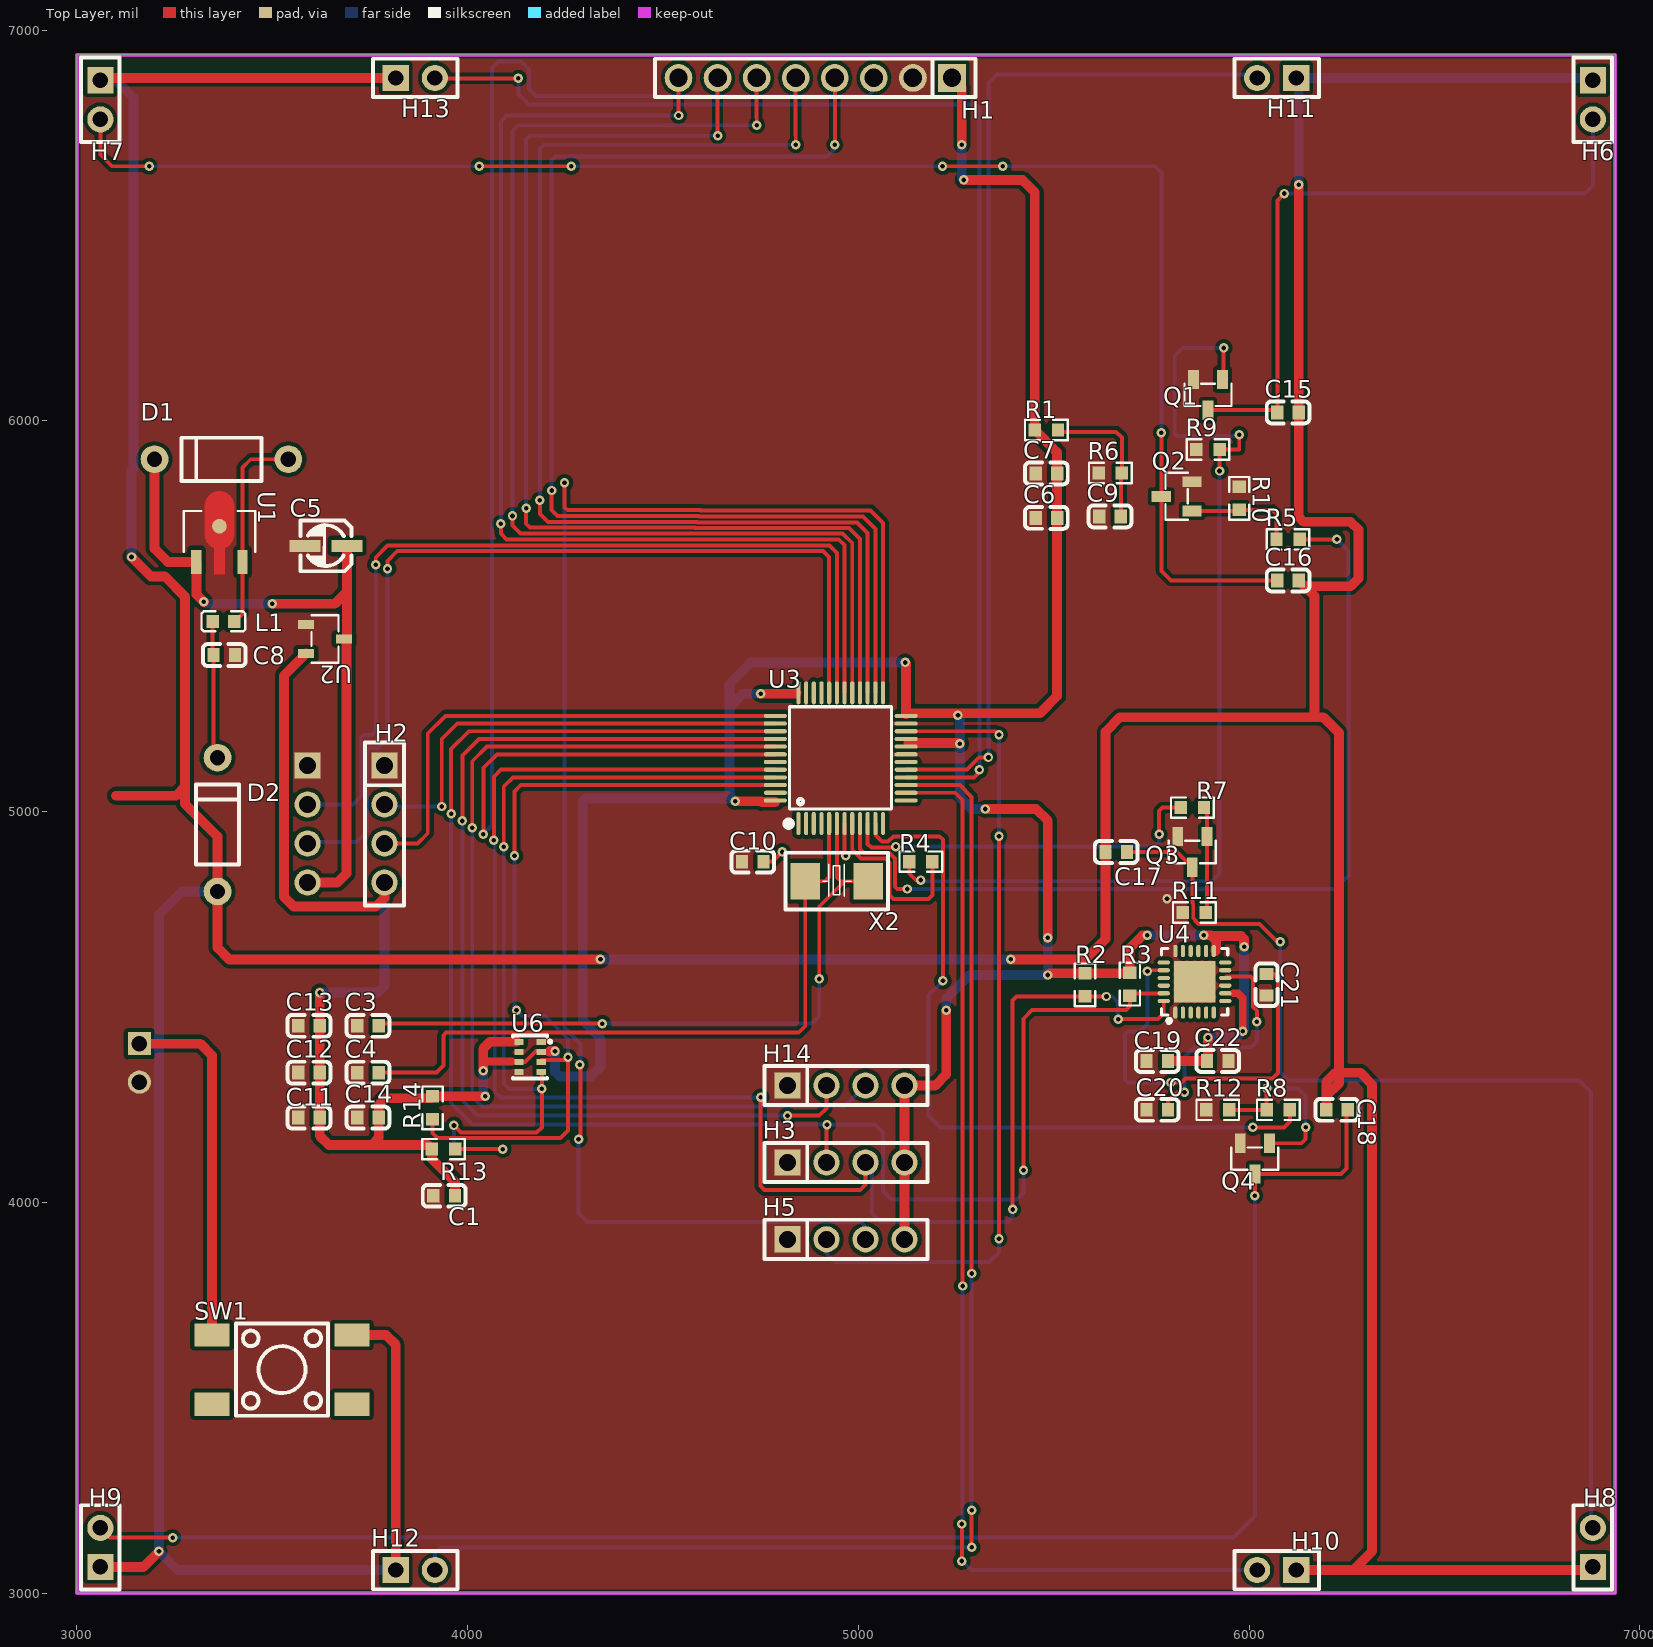
[diagram p0: Top Layer view]
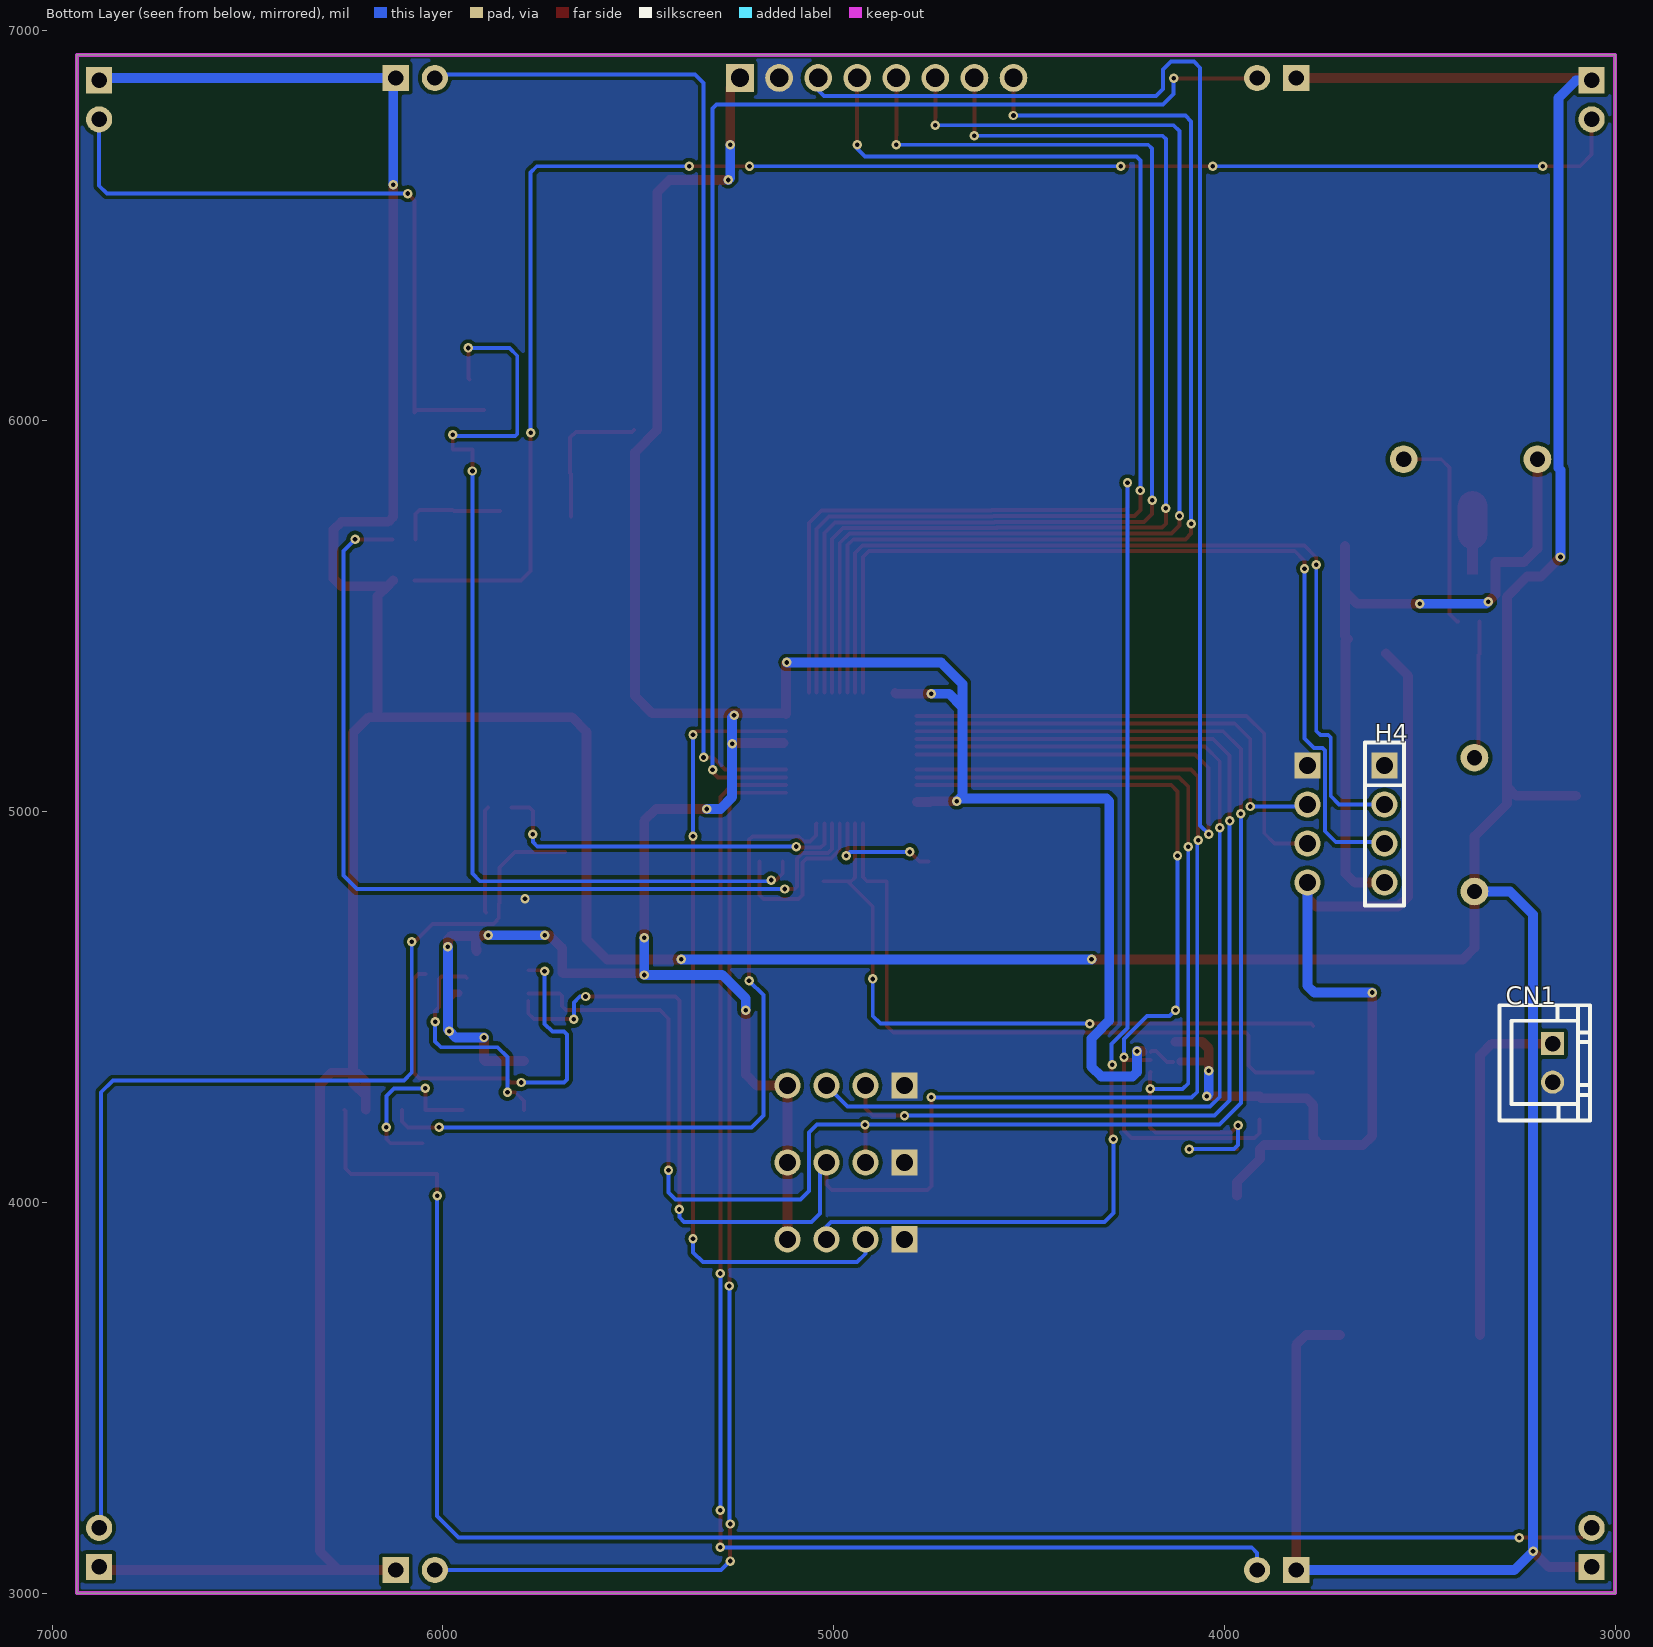
[diagram p1: Bottom Layer view, seen from below]
# Altium PCB MISC51791.pcbdoc
Units mil, origin at the board's own origin, x right, y up, seen from the top; angles counter-clockwise.
Board outline 3937.01 x 3937.01 mil, 2 copper layers (Top Layer, Bottom Layer), stack 62.206 mil thick; 64 components, 49 nets, 227 pads, 105 vias.

## Layer stack, top to bottom
Top Solder Mask Layer: solder mask 0.394, Dk 3.3
Top Layer: signal copper 1.379
Dielectric1: surface 59.449, FR4, Dk 4.5
Bottom Layer: signal copper 1.378
Bottom Solder Mask Layer: solder mask 0.394, Dk 3.3

## Board outline
3000,6937.01 3000,3000 6937.01,3000 6937.01,6937.01

## Design rules (kind name [scope] priority, off if disabled: settings)
BoardOutlineClearance copperThickness2oz_1 [All] p2 off: genericclearance=7.99 ignorepadtopadclearanceinfootprint=FALSE except(0: Arc-SplitContinuation Track-SplitContinuation SMDPad-SplitContinuation THPad-SplitContinuation Via-SplitContinuation Fill-SplitContinuation Region-SplitContinuation Poly-SplitContinuation Text-SplitContinuation Hole-SplitContinuation; 5.98: Arc-CutoutEdge SMDPad-CutoutEdge THPad-CutoutEdge Via-CutoutEdge Fill-CutoutEdge Region-CutoutEdge Text-CutoutEdge; 6.93: Hole-OutlineEdge Hole-CutoutEdge; 10: Poly-OutlineEdge Poly-CutoutEdge; 11.81: Arc-OutlineEdge Track-OutlineEdge SMDPad-OutlineEdge THPad-OutlineEdge Via-OutlineEdge Fill-OutlineEdge Region-OutlineEdge Text-OutlineEdge Track-CutoutEdge)
BoardOutlineClearance copperThickness1oz_1 [All] p4: genericclearance=4.02 ignorepadtopadclearanceinfootprint=FALSE except(0: Arc-SplitContinuation Track-SplitContinuation SMDPad-SplitContinuation THPad-SplitContinuation Via-SplitContinuation Fill-SplitContinuation Region-SplitContinuation Poly-SplitContinuation Text-SplitContinuation Hole-SplitContinuation; 6: SMDPad-CutoutEdge THPad-CutoutEdge Via-CutoutEdge Fill-CutoutEdge Region-CutoutEdge Text-CutoutEdge; 6.93: Hole-OutlineEdge Hole-CutoutEdge; 10: Poly-OutlineEdge Poly-CutoutEdge; 11.8: Arc-OutlineEdge Track-OutlineEdge SMDPad-OutlineEdge THPad-OutlineEdge Via-OutlineEdge Fill-OutlineEdge Region-OutlineEdge Text-OutlineEdge; 11.81: Arc-CutoutEdge Track-CutoutEdge)
Clearance copperThickness2oz [All] p1 off: gap=7.99 ignorepadtopadclearanceinfootprint=FALSE except(5.98: SMDPad-Track SMDPad-SMDPad THPad-Track SMDPad-THPad THPad-THPad Track-Via SMDPad-Via THPad-Via Via-Via Fill-Track Region-Track Fill-SMDPad Region-SMDPad Fill-THPad Region-THPad Fill-Via Region-Via Fill-Fill Fill-Region Region-Region Arc-Track Arc-SMDPad Arc-THPad Arc-Via Fill-Arc Region-Arc Arc-Arc Text-Track SMDPad-Text Text-THPad Text-Via Fill-Text Region-Text Arc-Text Text-Text; 6.93: Hole-Track Hole-SMDPad Hole-THPad Hole-Via Fill-Hole Region-Hole Hole-Arc Hole-Text; 10: Poly-Track Poly-SMDPad Poly-THPad Poly-Via Poly-Fill Poly-Region Poly-Poly Poly-Arc Poly-Text Poly-Hole)
Clearance copperThickness1oz [All] p3: gap=4.02 ignorepadtopadclearanceinfootprint=FALSE except(5.98: SMDPad-Track SMDPad-SMDPad THPad-Track SMDPad-THPad THPad-THPad Track-Via SMDPad-Via THPad-Via Via-Via Fill-Track Region-Track Fill-SMDPad Region-SMDPad Fill-THPad Region-THPad Fill-Via Region-Via Fill-Fill Fill-Region Region-Region; 6: Arc-Track Arc-SMDPad Arc-THPad Arc-Via Fill-Arc Region-Arc Arc-Arc Text-Track SMDPad-Text Text-THPad Text-Via Fill-Text Region-Text Arc-Text Text-Text; 6.93: Hole-Track Hole-SMDPad Hole-THPad Hole-Via Fill-Hole Region-Hole Hole-Arc Hole-Text; 10: Poly-Track Poly-SMDPad Poly-THPad Poly-Via Poly-Fill Poly-Region Poly-Poly Poly-Arc Poly-Text Poly-Hole)
DiffPairsRouting differentialPair [All] p1: maxlimit=6 minlimit=6 mostfreqgap=6 toplayer_minwidth=5 toplayer_prefwidth=10 toplayer_maxwidth=100 toplayer_mingap=6 toplayer_prefgap=6 toplayer_maxgap=6 bottomlayer_minwidth=5 bottomlayer_prefwidth=10 bottomlayer_maxwidth=100 bottomlayer_mingap=6 bottomlayer_prefgap=6 bottomlayer_maxgap=6 maxuncoupledlength=10
HoleToHoleClearance otherClearance [All] p1: gap=11.81 allowstackedmicrovias=TRUE
Length netLength [All] p1: minlimit=0 maxlimit=0
MatchedLengths netLengthTolerance [All] p1: tolerance=1000
PasteMaskExpansion pasteMaskExpansion [All] p1: expansion=0
PlaneConnect innerPlane [All] p1: planeconnectstyle=Relief reliefexpansion=20 reliefentries=4 reliefconductorwidth=10 reliefairgap=10
PolygonConnect "copperRegion_Top Layer" [(InNet('GND')) And OnLayer('Top Layer')] p1: connectstyle=Direct reliefconductorwidth=10 reliefentries=4 polygonreliefangle="90 Angle" airgapwidth=10 via.connectstyle=Relief via.reliefconductorwidth=10 via.reliefentries=4 via.polygonreliefangle="90 Angle" via.airgapwidth=10
PolygonConnect "copperRegion_Bottom Layer" [(InNet('GND')) And OnLayer('Bottom Layer')] p2: connectstyle=Direct reliefconductorwidth=10 reliefentries=4 polygonreliefangle="90 Angle" airgapwidth=10 via.connectstyle=Relief via.reliefconductorwidth=10 via.reliefentries=4 via.polygonreliefangle="90 Angle" via.airgapwidth=10
PolygonConnect copperRegion [(InNet('GND'))] p3: connectstyle=Direct reliefconductorwidth=10 reliefentries=4 polygonreliefangle="90 Angle" airgapwidth=10 via.connectstyle=Relief via.reliefconductorwidth=10 via.reliefentries=4 via.polygonreliefangle="90 Angle" via.airgapwidth=10
RoutingVias viaSize [All] p1: holewidth=12.01 width=24.02 viastyle="Through Hole" minholewidth=11.81 minwidth=19.68 maxholewidth=248.03 maxwidth=393.7
SolderMaskExpansion solderMaskExpansion [IsVia] p1: expansion=-1000 istentingtop=TRUE
SolderMaskExpansion solderMaskExpansion [All] p2: expansion=2 istentingtop=FALSE
Width copperThickness2oz_2 [All] p1 off: maxlimit=100 minlimit=8 preferedwidth=10
Width copperThickness1oz_2 [All] p2: maxlimit=100 minlimit=5 preferedwidth=10

## Components (designator, comment, footprint, x,y, rotation, side; value= is the part's Value field where it differs from the comment)
C1 "100nF" C0603 3940,4017.01 r0 top
C3 "20pF" C0603 3745,4452.01 r0 top
C4 "20pF" C0603 3745,4332.01 r0 top
C5 "0.1uF" C_Ele_SMD_3x5.4mm 3637.34,5680.81 r0 top
C6 "0.1uF" C0603 5481.33,5752.01 r0 top
C7 "0.1uF" C0603 5481.33,5865.81 r0 top
C8 "0.1uF" C0603 3377.29,5400.81 r180 top
C9 "22pF" C0603 5644.34,5755.81 r0 top
C10 "0.1uF" C0603 4730,4872.01 r0 top
C11 "0.1uF" C0603 3593.97,4217.01 r0 top
C12 "0.1uF" C0603 3593.97,4332.15 r0 top
C13 "0.1uF" C0603 3593.97,4452.01 r0 top
C14 "0.1uF" C0603 3745,4217.01 r0 top
C15 "0.1uF" C0603 6100,6022.01 r0 top
C16 "0.1uF" C0603 6100,5592.01 r0 top
C17 "0.1uF" C0603 5660,4897.01 r180 top
C18 "0.1uF" C0603 6225,4237.01 r180 top
C19 "10nF" C0603 5765.21,4361.95 r0 top
C20 "0.1uF" C0603 5765,4237.01 r0 top
C21 "2.2nF" C0603 6045,4557.01 r270 top
C22 "0.1uF" C0603 5920,4362.01 r0 top
CN1 "HX-XH2.54-2PZZ" CONN-TH_2P-P2.50_HX-2.54MM-2P-ZZ-MS 3160,4357.01 r270 bottom
D1 "" DO_1N4007 3370,5902.01 r0 top
D2 "" DO_1N4007 3360,4967.01 r270 top
H1 "" HDR-TH_8P-P2.54-V-F-1 4889.76,6877.95 r180 top
H2 "" HDR-TH_4P-P2.54-V-F 3787.4,4968.5 r270 top
H3 "" HDR-TH_4P-P2.54-V-F 4968.5,4102.38 r0 top
H4 "" HDR-TH_4P-P2.54-V-F 3590.55,4968.5 r270 bottom
H5 "" HDR-TH_4P-P2.54-V-F 4968.5,3905.53 r0 top
H6 "" HDR-TH_2P-P2.54-V-F 6880,6822.01 r270 top
H7 "" HDR-TH_2P-P2.54-V-F 3060,6822.01 r270 top
H8 "" HDR-TH_2P-P2.54-V-F 6880,3117.01 r90 top
H9 "" HDR-TH_2P-P2.54-V-F 3060,3117.01 r90 top
H10 "" HDR-TH_2P-P2.54-V-F 6070.86,3059.07 r180 top
H11 "" HDR-TH_2P-P2.54-V-F 6070.87,6877.95 r180 top
H12 "" HDR-TH_2P-P2.54-V-F 3866.14,3059.06 r0 top
H13 "" HDR-TH_2P-P2.54-V-F 3866.14,6877.95 r0 top
H14 "" HDR-TH_4P-P2.54-V-F 4968.5,4299.21 r0 top
L1 "47uH" L0603 3375,5487.01 r0 top
Q1 "" SOT-23-3_L2.9-W1.3-P1.90-LS2.4-BR 5895,6067.01 r90 top
Q2 "" SOT-23-3_L2.9-W1.3-P1.90-LS2.4-BR 5815,5807.01 r0 top
Q3 "" SOT-23-3_L2.9-W1.3-P1.90-LS2.4-BR 5855,4897.01 r90 top
Q4 "" SOT-23-3_L2.9-W1.3-P1.90-LS2.4-BR 6015,4112.01 r90 top
R1 "100R" R0603 5481.33,5977.01 r180 top
R2 "4.7K" R0603 5580,4557.01 r90 top
R3 "4.7K" R0603 5694.92,4558.62 r90 top
R4 "100R" R0603 5160,4872.01 r0 top locked
R5 "100R" R0603 6100,5697.01 r0 top
R6 "100R" R0603 5645,5867.01 r0 top
R7 "100R" R0603 5855.02,5010.49 r180 top
R8 "100R" R0603 6075,4237.01 r0 top
R9 "10K" R0603 5895,5927.01 r0 top
R10 "10K" R0603 5975,5802.01 r270 top
R11 "10K" R0603 5860,4742.01 r0 top
R12 "10K" R0603 5920,4237.01 r0 top
R13 "4.7K" R0603 3938.37,4136.44 r180 top
R14 "4.7K" R0603 3910,4242.01 r90 top
SW1 "KH-6X6X5H-STM" SW-SMD_4P-L6.0-W6.0-P4.50-LS9.0_H5.0 3525,3572.01 r0 top
U1 "78L05" SOT-89-3_L4.5-W2.5-P1.50-LS4.2-BR 3364.91,5692.7 r270 top
U2 "XC6206P332MR-G" SOT-23-3_L2.9-W1.6-P1.90-LS2.8-BR 3635,5442.01 r180 top
U3 "STM32G474CBT6" LQFP-48_L7.0-W7.0-P0.50-LS9.0-BL 4955,5137.01 r0 top locked
U4 "MPU-6050" QFN-24_L4.0-W4.0-P0.50-BL-EP2.7 5860.53,4564.7 r0 top
U6 "BMP280" LGA-8_L2.5-W2.0-P0.65_AMP6127 4160,4372.01 r0 top
X2 "8MHz" CRYSTAL-SMD_L5.0-W3.2 4945,4822.01 r180 top

## Footprints (in the part's own frame and the unit in brackets; to place one, negate y for a bottom-side part, rotate by r counter-clockwise, add the part's x,y. Pads: shape width x height; smd on the part's side, far side on the other; paste and mask are expansions set on the pad)
C0603 [mm]
  rect 0.8x0.9 smd: 1(-0.7,0) 2(0.7,0)
  silkscreen extent -1.39,-0.71 1.39,0.71
C_Ele_SMD_3x5.4mm [mil]
  rect 78.7x31.5 smd paste+0 mask+2: 1(54.1,-0.55) 2(-53.7,-0.55)
  silkscreen extent -65,-65 65,65
CONN-TH_2P-P2.50_HX-2.54MM-2P-ZZ-MS [mm]
  rect 1.5x1.5 hole 1: 1(-1.25,0)
  round 1.5 hole 1: 2(1.25,0)
  silkscreen extent -3.75,-3.46 3.75,2.44
CRYSTAL-SMD_L5.0-W3.2 [mm]
  rect 1.9x2.4 smd: 1(-2.05,0) 2(2.05,0)
  silkscreen extent -3.32,-1.85 3.33,1.85
DO_1N4007 [mm]
  round 1.8 hole 1 paste+0 mask+0.051: 1(-4.35,0) 2(4.35,0)
  silkscreen extent -2.6,-1.4 2.6,1.4
HDR-TH_2P-P2.54-V-F [mm]
  rect 1.7x1.7 hole 1: 1(-1.27,0)
  round 1.7 hole 1: 2(1.27,0)
  silkscreen extent -2.74,-1.25 2.74,1.25
HDR-TH_4P-P2.54-V-F [mm]
  rect 1.7x1.7 hole 1.1: 1(-3.81,0)
  round 1.7 hole 1.1: 2(-1.27,0) 3(1.27,0) 4(3.81,0)
  silkscreen extent -5.29,-1.27 5.29,1.27
HDR-TH_8P-P2.54-V-F-1 [mm]
  rect 1.8x1.8 hole 1.2: 1(-8.89,0)
  round 1.8 hole 1.2: 2(-6.35,0) 3(-3.81,0) 4(-1.27,0) 5(1.27,0) 6(3.81,0) 7(6.35,0) 8(8.89,0)
  silkscreen extent -10.41,-1.25 10.41,1.25
L0603 [mm]
  rect 0.8x0.864 smd paste-100 mask+0.051: 1(-0.7,0) 2(0.7,0)
  silkscreen extent -1.42,-0.65 1.42,0.65
LGA-8_L2.5-W2.0-P0.65_AMP6127 [mm]
  rect 0.6x0.4 smd: 1(0.725,0.975) 2(0.725,0.325) 3(0.725,-0.325) 4(0.725,-0.975) 5(-0.725,-0.975) 6(-0.725,-0.325) 7(-0.725,0.325) 8(-0.725,0.975)
  silkscreen extent -1.1,-1.4 1.4,1.4
LQFP-48_L7.0-W7.0-P0.50-LS9.0-BL [mm]
  oval 0.27x1.5 smd paste+0 mask+0.05: 1(-2.75,-4.25) 2(-2.25,-4.25) 3(-1.75,-4.25) 4(-1.25,-4.25) 5(-0.75,-4.25) 6(-0.25,-4.25) 7(0.25,-4.25) 8(0.75,-4.25) 9(1.25,-4.25) 10(1.75,-4.25) 11(2.25,-4.25) 12(2.75,-4.25) 25(2.75,4.25) 26(2.25,4.25) 27(1.75,4.25) 28(1.25,4.25) 29(0.75,4.25) 30(0.25,4.25) 31(-0.25,4.25) 32(-0.75,4.25) 33(-1.25,4.25) 34(-1.75,4.25) 35(-2.25,4.25) 36(-2.75,4.25)
  oval 1.5x0.27 smd paste+0 mask+0.05: 13(4.25,-2.75) 14(4.25,-2.25) 15(4.25,-1.75) 16(4.25,-1.25) 17(4.25,-0.75) 18(4.25,-0.25) 19(4.25,0.25) 20(4.25,0.75) 21(4.25,1.25) 22(4.25,1.75) 23(4.25,2.25) 24(4.25,2.75) 37(-4.25,2.75) 38(-4.25,2.25) 39(-4.25,1.75) 40(-4.25,1.25) 41(-4.25,0.75) 42(-4.25,0.25) 43(-4.25,-0.25) 44(-4.25,-0.75) 45(-4.25,-1.25) 46(-4.25,-1.75) 47(-4.25,-2.25) 48(-4.25,-2.75)
  silkscreen extent -3.59,-4.46 3.3,3.34
QFN-24_L4.0-W4.0-P0.50-BL-EP2.7 [mm]
  oval 0.28x0.8 smd paste-100 mask+0.05: 1(-1.25,-2) 2(-0.75,-2) 3(-0.25,-2) 4(0.25,-2) 5(0.75,-2) 6(1.25,-2) 13(1.25,2) 14(0.75,2) 15(0.25,2) 16(-0.25,2) 17(-0.75,2) 18(-1.242,2)
  oval 0.8x0.28 smd paste-100 mask+0.05: 7(2,-1.25) 8(2,-0.75) 9(2,-0.25) 10(2,0.25) 11(2,0.75) 12(2,1.25) 19(-2,1.25) 20(-2,0.75) 21(-2,0.25) 22(-2,-0.25) 23(-2,-0.75) 24(-2,-1.25)
  rect 2.7x2.7 smd paste-100 mask+0.05: 25(0.012,0)
  silkscreen extent -2.14,-2.79 2.16,2.15
R0603 [mil]
  rect 31.75x34.02 smd paste-3937.01 mask+2: 1(-29.66,0) 2(29.66,0)
  silkscreen extent -55,-26 55,26
SOT-23-3_L2.9-W1.3-P1.90-LS2.4-BR [mm]
  rect 1.25x0.7 smd: 1(1,-0.95) 2(1,0.95) 3(-1,0)
  silkscreen extent -0.73,-1.53 0.73,1.53
SOT-23-3_L2.9-W1.6-P1.90-LS2.8-BR [mm]
  rect 1.07x0.6 smd: 1(1.235,-0.95) 2(1.235,0.95) 3(-1.235,0)
  silkscreen extent -0.88,-1.54 0.88,1.54
SOT-89-3_L4.5-W2.5-P1.50-LS4.2-BR [mm]
  rect 1.575x0.672 smd: 1(1.356,-1.5) 3(1.356,1.5)
  round 0.95 smd: 2(-0.966,0)
  Top Layer region: -2.283,0.95 -0.429,0.95 -0.384,0.949 -0.34,0.946 -0.296,0.94 -0.252,0.933 -0.208,0.924 -0.165,0.912 -0.123,0.899 -0.081,0.884 -0.04,0.866 0,0.847 0.04,0.826 0.078,0.803 0.115,0.779 0.151,0.752 0.185,0.724 0.219,0.695 0.251,0.664 0.281,0.631 0.31,0.597 0.337,0.562 0.362,0.525 0.386,0.488 0.408,0.449 0.428,0.409 0.447,0.33 2.144,0.33 2.144,-0.33 0.447,-0.33 0.428,-0.409 0.408,-0.449 0.386,-0.488 0.362,-0.526 0.337,-0.562 0.31,-0.597 0.281,-0.631 0.251,-0.664 0.219,-0.695 0.185,-0.725 0.151,-0.753 0.115,-0.779 0.078,-0.804 0.04,-0.827 0,-0.848 -0.04,-0.867 -0.081,-0.884 -0.123,-0.899 -0.165,-0.913 -0.208,-0.924 -0.252,-0.934 -0.296,-0.941 -0.34,-0.946 -0.384,-0.949 -0.429,-0.95 -2.283,-0.95 -2.328,-0.949 -2.372,-0.946 -2.416,-0.941 -2.46,-0.934 -2.504,-0.924 -2.547,-0.913 -2.589,-0.899 -2.631,-0.884 -2.672,-0.867 -2.713,-0.848 -2.752,-0.827 -2.79,-0.804 -2.827,-0.779 -2.863,-0.753 -2.898,-0.725 -2.931,-0.695 -2.963,-0.664 -2.993,-0.631 -3.022,-0.597 -3.049,-0.562 -3.075,-0.526 -3.098,-0.488 -3.12,-0.449 -3.141,-0.409 -3.159,-0.369 -3.175,-0.327 -3.189,-0.285 -3.202,-0.242 -3.212,-0.199 -3.22,-0.155 -3.227,-0.111 -3.231,-0.067 -3.233,-0.022 -3.233,0.022 -3.231,0.067 -3.227,0.111 -3.22,0.155 -3.212,0.199 -3.202,0.242 -3.189,0.285 -3.175,0.327 -3.159,0.369 -3.141,0.409 -3.12,0.449 -3.098,0.488 -3.075,0.525 -3.049,0.562 -3.022,0.597 -2.993,0.631 -2.963,0.664 -2.931,0.695 -2.898,0.724 -2.863,0.752 -2.827,0.779 -2.79,0.803 -2.752,0.826 -2.713,0.847 -2.672,0.866 -2.631,0.884 -2.589,0.899 -2.547,0.912 -2.504,0.924 -2.46,0.933 -2.416,0.94 -2.372,0.946 -2.328,0.949
  silkscreen extent -1.95,-2.33 0.7,2.33
SW-SMD_4P-L6.0-W6.0-P4.50-LS9.0_H5.0 [mm]
  rect 2.3x1.5 smd: 1(-4.55,2.25) 2(4.55,2.25) 3(-4.55,-2.25) 4(4.55,-2.25)
  silkscreen extent -3,-3 3,3

## Via types
v1: diameter 24.02, hole 12, Top Layer to Bottom Layer, 105 vias

## Nets (pads, with @x,y where several pads share a name; then routed paths per layer and width w, separated by ;. In a path a pad name is that pad's centre, name@x,y a point inside that pad or via, vN(x,y) a via of type N, cw(c..) or ccw(c..) an arc to the next point about the centre after c; other vN are vias at no path point)
3.3V: C1.2 C6.2 C7.2 C11.2 C12.2 C13.2 C14.2 C19.2 C22.1 H1.1 H2.4 H3.4 H5.4 H14.4 R1.2 R2.2 R3.2 R13.2 R14.2 U2.2 U3.20 U3.21 U3.24 U3.36 U3.48 U4.8 U4.13 U6.2 U6.6 U6.8 | length 10851.4
  Top Layer w10: U6.6 4147.21,4359.22 4175,4387.01 4186.33,4387.01 U6.2 ; C22.1 C22.1@5895,4364.57
  Top Layer w20: 4040,4358.91 4042.03,4360.94 4112.96,4360.94 ; 5960.22,4535.17 5971.83,4535.17 5983.79,4523.22 v1(5983.79,4438.22)
  Top Layer w25: U2.2 3530,5348.23 3530,4782.01 3555,4757.01 3765,4757.01 3787.4,4779.41 H2.4 ; v1(3621.53,4537.01) C13.2 C12.2 C11.2 3621.53,4170.47 3645,4147.01 3755,4147.01 ; C1.2 3967.56,4052.36 3908.71,4111.21 R13.2 3898.14,4147.01 3755,4147.01 ; v1@4040,4271.67 R14.2 3905,4266.67 3789.66,4266.67 3772.56,4249.57 C14.2 3772.56,4164.57 3755,4147.01 ; v1(4040,4337.01) 4040,4358.91 4040,4393.48 4057.68,4411.16 U6.8@4125.18,4411.16 ; 4209.65,4385.68 4211.18,4387.21 v1(4223.8,4387.21) ; v1(4685,5027.01) 4751.23,5027.01 4753.61,5024.63 U3.48@4787.68,5024.63 ; v1(4750,5302.01) 4840.3,5302.01 U3.36@4842.62,5304.33 ; H5.4 H3.4 H14.4 5197.2,4299.21 5225,4327.01 v1(5225,4492.01) ; v1(5120,5382.01) 5122.32,5379.69 U3.24@5122.32,5250.28 ; U3.24@5122.32,5249.39 U3.24@5122.32,5250.28 ; 5128.44,5175.99 5257.62,5175.99 v1(5260,5173.61) ; H1.1 5265,6852.72 v1(5265,6707.01) ; v1(5270,6617.01) 5420,6617.01 5451.67,6585.34 R1.2 5508.89,5919.79 C7.2 C6.2 5508.89,5295.9 5465,5252.01 5260,5252.01 v1(5255,5247.01) 5250,5252.01 5124.05,5252.01 U3.24@5122.32,5250.28 ; v1(5325,5007.01) 5455,5007.01 5485,4977.01 v1(5485,4677.01) ; v1(5485,4582.01) 5489.66,4586.67 R2.2 5693.31,4586.67 R3.2 5694.92,4651.58 5726.82,4683.48 v1(5739.61,4683.48) ; C19.2 C22.1 ; v1(5884.09,4683.48) 5903.52,4683.48 5909.74,4677.27 ; C22.1@5895,4364.57 v1(5895,4422.01) ; U4.13@5914.06,4643.44 5914.06,4647.76 5915.97,4649.67 5915.97,4671.03 5909.74,4677.27 ; v1(5987.5,4654.51) 5987.5,4674.51 5980,4682.01 5914.48,4682.01 5909.74,4677.27
  Bottom Layer w25: v1(3621.53,4537.01) 3770,4537.01 3787.4,4554.41 H2.4 ; v1(4040,4337.01) 4040,4276.67 v1(4045,4271.67) ; v1(4223.8,4387.21) 4223.8,4333.21 4235,4322.01 4315,4322.01 4340,4347.01 4340,4419.37 4314.51,4444.86 4314.51,4446.27 4295,4465.78 4295,5027.01 4302.07,5034.08 v1@4677.93,5034.08 ; v1(4685,5027.01) v1@4677.93,5034.08 ; v1(4750,5302.01) 4705,5302.01 4671.08,5268.09 4670,5268.09 ; v1(5120,5382.01) 4725,5382.01 4670,5327.01 4670,5268.09 ; v1(5225,4492.01) 5225,4522.01 5285,4582.01 v1(5485,4582.01) v1(5485,4677.01) ; v1(5255,5247.01) 5260,5242.01 v1(5260,5173.61) 5260,5037.01 5290,5007.01 v1(5325,5007.01) ; v1(5265,6707.01) 5265,6622.01 v1(5270,6617.01) ; v1(5739.61,4683.48) v1(5884.09,4683.48) ; v1(5895,4422.01) 5967.57,4422.01 v1(5983.79,4438.22) 5987.5,4441.93 v1(5987.5,4654.51) ; 4670,5268.09 4670,5042.01 v1@4677.93,5034.08
$1N3: C8.2 D2.1 L1.1 | length 353.9
  Top Layer w10: L1.1 3347.45,5403.1 C8.2 3349.73,5148.53 D2.1
$1N6: D1.2 L1.2 U1.3 | length 530.3
  Top Layer w10: L1.2 3405,5487.01 3423.96,5505.97 U1.3 3423.96,5880.97 3445,5902.01 D1.2
$1N10: C9.2 R1.1 R6.2 | length 374.5
  Top Layer w10: R1.1 5515.99,5972.01 5660,5972.01 5674.66,5957.35 R6.2 5671.9,5864.25 C9.2
$1N18: C10.2 U3.7 | length 309.3
  Top Layer w10: C10.2 4780,4872.01 v1(4805,4897.01) ; U3.7 4964.84,4890.21 v1(4968.15,4886.9)
  Bottom Layer w10: v1(4805,4897.01) 4958.04,4897.01 v1(4968.15,4886.9)
$1N84: C15.1 H6.2 Q1.3 | length 1715.3
  Top Layer w10: Q1.3 6066.81,6027.64 C15.1 6072.44,6564.45 v1(6090,6582.01)
  Bottom Layer w10: v1(6090,6582.01) 6860,6582.01 6880,6602.01 H6.2
$1N86: Q1.1 R4.1 R9.2 | length 2597.8
  Top Layer w10: R4.1 5130.34,4841.67 5147.01,4825 v1(5160,4825) ; v1(5924.66,5872.01) R9.2 5975,5927.01 v1(5975,5964.94) ; Q1.1 5935,6108.98 v1(5935,6187.01)
  Bottom Layer w10: v1(5160,4825) 5162.99,4822.01 5905,4822.01 5924.66,4841.67 v1(5924.66,5872.01) ; v1(5935,6187.01) 5830,6187.01 5810,6167.01 5810,5967.01 5815,5962.01 5972.07,5962.01 v1(5975,5964.94)
$1N89: Q2.1 R5.1 R10.2 | length 286.2
  Top Layer w10: Q2.1 5972.26,5769.61 R10.2 6059.66,5772.35 6070.34,5761.67 R5.1
$1N91: C16.1 H7.2 Q2.3 | length 4151.4
  Top Layer w10: H7.2 3060,6682.01 3090,6652.01 v1(3185,6652.01) ; v1(4030,6652.01) v1(4265,6652.01) ; v1(5215.44,6652.01) v1(5370,6652.01) ; v1(5775.63,5970.18) Q2.3 5775.63,5616.38 5800,5592.01 C16.1
  Bottom Layer w10: v1(3185,6652.01) v1(4030,6652.01) ; v1(4265,6652.01) v1(5215.44,6652.01) ; v1(5370,6652.01) 5760,6652.01 5775.63,6636.38 v1(5775.63,5970.18)
$1N94: Q3.1 R7.1 R11.2 | length 272.8
  Top Layer w10: R7.1 5892.4,5002.77 Q3.1 5892.4,4744.75 R11.2
$1N96: C17.1 H8.2 Q3.3 | length 2831.3
  Top Layer w10: C17.1 5815.63,4897.01 Q3.3 5855,4765.77 5857.2,4763.57 5857.2,4727.83 5862.8,4722.23 5862.8,4720.45 5871.02,4712.23 6027.29,4712.23 6072.52,4667.01 v1(6080,4667.01)
  Bottom Layer w10: v1(6080,4667.01) 6080,4332.01 6100,4312.01 6845,4312.01 6875,4282.01 6875,3172.01 H8.2
$1N99: Q4.1 R8.1 R12.2 | length 466.1
  Top Layer w10: R12.2 R8.1 6045,4237.35 v1(6045,4292.01) ; Q4.1 6134.37,4151.38 6145,4162.01 v1(6145,4192.01)
  Bottom Layer w10: v1(6045,4292.01) 6125,4292.01 6145,4272.01 v1(6145,4192.01)
$1N101: C18.1 H9.2 Q4.3 | length 4255.8
  Top Layer w10: H9.2 3085,3142.01 v1(3245,3142.01) ; v1(6015,4017.01) Q4.3 6235.63,4072.64 6250,4087.01 6250,4234.45 C18.1
  Bottom Layer w10: v1(3245,3142.01) 5960,3142.01 6015,3197.01 v1(6015,4017.01)
$1N107: C20.2 U4.10 | length 604.4
  Top Layer w10: C20.2 5792.56,4259.57 5815,4282.01 v1(5835,4282.01) ; U4.10 5942.46,4577.73 6004.28,4577.73 6010,4572.01 6010,4500.45 6020,4490.45 v1(6020,4462.01)
  Bottom Layer w10: v1(5835,4282.01) 5835,4372.01 5860,4397.01 6005,4397.01 6020,4412.01 v1(6020,4462.01)
$1N110: C21.1 U4.20 | length 1041.3
  Top Layer w10: v1(5740,4592.01) 5744.85,4592.01 5747.07,4594.23 U4.20 ; v1(5800,4307.01) 5827.48,4307.01 5837.48,4317.01 6060,4317.01 6073.7,4330.71 6073.7,4573.31 6062.44,4584.57 C21.1
  Bottom Layer w10: v1(5740,4592.01) 5740,4457.01 5720,4437.01 5690,4437.01 5682.93,4429.94 5682.93,4314.08 5690,4307.01 v1(5800,4307.01)
$1N126: C4.2 U3.5 X2.2 | length 1759.8
  Top Layer w10: C4.2 3920,4332.01 3937.93,4349.94 3937.93,4427.19 3945.24,4434.5 4847.49,4434.5 4864.29,4451.3 X2.2 4915,4822 4925.47,4832.48 U3.5
$1N129: C3.2 U3.6 X2.1 | length 1793.2
  Top Layer w10: C3.2 3778.04,4457.49 v1(4345,4457.49) ; v1(4900,4572.01) 4900,4757.54 4964.47,4822 X2.1 4955,4822.01 4945.16,4831.85 U3.6
  Bottom Layer w10: v1(4345,4457.49) 4880.48,4457.49 4900,4477.01 v1(4900,4572.01)
+5V: C5.1 D1.1 H4.4 U1.1 U2.3 | length 1794.4
  Top Layer w25: D1.1 3198.74,5673.27 3232.7,5639.31 U1.1 3305.85,5556.16 v1(3325,5537.01) ; v1(3500,5532.01) 3660,5532.01 3683.62,5555.63 ; H4.4 3666.5,4818.5 3690,4842.01 3690,5435.63 U2.3 3691.05,5449.43 3691.05,5555.63 3683.62,5555.63 ; C5.1 3691.44,5563.45 3683.62,5555.63
  Bottom Layer w25: v1(3325,5537.01) 3330,5532.01 v1(3500,5532.01)
CE: H1.3 U3.42 | length 3990.3
  Top Layer w10: v1(4040.1,4942.4) 4040.49,4942.79 4040.49,5112.5 4074.84,5146.85 U3.42
  Bottom Layer w10: v1(4040.1,4942.4) 4062.01,4964.31 4062.01,6904.02 4078.2,6920.21 4136.8,6920.21 4157.56,6899.45 4157.56,6849.45 4175.47,6831.54 5024.53,6831.54 5039.76,6846.77 H1.3
CSN: H1.4 U3.26 | length 3081.3
  Top Layer w10: v1(4215,5822.01) 4215,5772.01 4230,5757.01 4590.9,5757.01 4592.87,5755.04 5011.97,5755.04 5043.58,5723.43 U3.26 ; H1.4 4940,6877.72 v1(4940,6707.01)
  Bottom Layer w10: v1(4215,5822.01) 4215,6667.01 4225,6677.01 4920,6677.01 4940,6697.01 v1(4940,6707.01)
GND: C1.1 C3.1 C4.1 C5.2 C6.1 C7.1 C8.1 C9.1 C10.1 C11.1 C12.1 C13.1 C14.1 C19.1 C20.1 C21.2 C22.2 CN1.2 H1.2 H2.1 H3.1 H4.1 H5.1 H14.1 Q1.2 Q2.2 Q3.2 Q4.2 R6.1 R9.1 R10.1 R11.1 R12.1 U1.2 U2.1 U3.19 U3.23 U3.35 U3.47 U4.1 U4.9 U4.11 U4.18 U4.25 U6.1 U6.5 U6.7
  other v1: 5790,4777.01
IRQ: H1.8 U3.30 | length 2882.3
  Top Layer w10: v1(4085,5737.01) 4085,5712.01 4100,5697.01 4950,5697.01 4964.84,5682.17 U3.30 ; H1.8 4539.76,6806.77 4540,6806.54 v1(4540,6782.01)
  Bottom Layer w10: v1(4085,5737.01) 4085,6767.01 4100,6782.01 v1(4540,6782.01)
LED_PWM1: H10.2 U3.14 | length 2866.5
  Top Layer w10: U3.14 5248.58,5048.43 5267.01,5030 v1(5267.01,3786.07) ; v1(5265,3082.01) v1(5265,3177.01)
  Bottom Layer w10: v1(5265,3082.01) 5287.94,3059.07 H10.2 ; v1(5265,3177.01) 5267.01,3179.02 v1(5267.01,3786.07)
LED_PWM2: H11.2 U3.17 | length 2650.5
  Top Layer w10: U3.17 5277.95,5107.48 5309.34,5138.87 v1(5332.99,5138.87)
  Bottom Layer w10: v1(5332.99,5138.87) 5332.99,6865 5355,6887.01 6011.81,6887.01 H11.2
LED_PWM3: H12.2 U3.15 | length 3524.9
  Top Layer w10: U3.15 5260,5068.11 5290,5038.11 v1(5290,3817.89) ; v1(5290,3117.01) v1(5290,3212.01)
  Bottom Layer w10: H12.2 3916.14,3103.15 3930,3117.01 v1(5290,3117.01) ; v1(5290,3212.01) v1(5290,3817.89)
LED_PWM4: H13.2 U3.16 | length 3341.1
  Top Layer w10: H13.2 3917.09,6877.01 v1(4130,6877.01) ; U3.16 5295.79,5087.8 5310,5102.01 v1(5310,5107.01)
  Bottom Layer w10: v1(4130,6877.01) 4130,6837.01 4157.01,6810 5300,6810 5310,6800 v1(5310,5107.01)
MISO: H1.7 U3.28 | length 2890.3
  Top Layer w10: v1(4150,5777.01) 4150,5737.01 4160,5727.01 4581.53,5727.01 4582.51,5726.02 4975.98,5726.02 5004.21,5697.8 U3.28 ; H1.7 4639.76,6746.77 4640,6746.54 v1(4640,6730)
  Bottom Layer w10: v1(4150,5777.01) 4150,6722.01 4157.99,6730 v1(4640,6730)
MOSI: H1.6 U3.29 | length 3033.4
  Top Layer w10: v1(4115,5757.01) 4115,5732.01 4135,5712.01 4960,5712.01 4984.53,5687.48 U3.29 ; H1.6 4739.76,6776.77 4740,6776.54 v1(4740,6757.01)
  Bottom Layer w10: v1(4115,5757.01) 4115,6742.01 4130,6757.01 v1(4740,6757.01)
PWM1: R4.2 U3.8 | length 462.1
  Top Layer w10: U3.8 4984.53,4903.04 5007.33,4880.23 5070,4880.23 5080,4870.23 5080,4787.01 5090,4777.01 5180,4777.01 5189.66,4786.67 R4.2
PWM2: R5.2 U3.9 | length 2383
  Top Layer w10: U3.9 5004.21,4904.25 5014.21,4894.25 5079.79,4894.25 5094.02,4880.02 5094.02,4807.99 5100,4802.01 v1(5125,4802.01) ; R5.2 v1(6225,5697.01)
  Bottom Layer w10: v1(5125,4802.01) 6220,4802.01 6255,4837.01 6255,5667.01 v1(6225,5697.01)
PWM3: R7.2 U3.10 | length 946.5
  Top Layer w10: U3.10 5023.9,4917.76 5033.39,4908.26 5093.33,4908.26 v1(5095.81,4910.75) ; v1(5770,4942.01) 5770,5002.01 5778.48,5010.49 R7.2
  Bottom Layer w10: v1(5095.81,4910.75) 5758.74,4910.75 5770,4922.01 v1(5770,4942.01)
PWM4: R8.2 U3.11 | length 1913.1
  Top Layer w10: U3.11 5045,4968.27 5045,4939.56 5060.82,4923.74 5076.29,4923.74 5089.56,4937.01 5208.16,4937.01 5216.58,4928.59 v1(5216.58,4567.01) ; v1(6010,4192.01) 6090,4192.01 6104.66,4206.67 R8.2
  Bottom Layer w10: v1(5216.58,4567.01) 5180,4530.43 5180,4222.01 5210,4192.01 v1(6010,4192.01)
SCK: H1.5 U3.27 | length 3033.1
  Top Layer w10: v1(4185,5797.01) 4185,5762.01 4205.98,5741.02 4587.34,5741.02 4588.32,5740.04 4996.97,5740.04 5023.9,5713.11 U3.27 ; H1.5 4839.76,6731.77 4840,6731.54 v1(4840,6707.01)
  Bottom Layer w10: v1(4185,5797.01) 4185,6697.01 4195,6707.01 v1(4840,6707.01)
SCL1: H3.2 R3.1 U3.39 U4.23 | length 4361.2
  Top Layer w10: v1(3958.03,4995.04) 3958.03,5160.04 4003.9,5205.91 U3.39 ; H3.2 4918.5,4188.51 4920,4190 v1(4920,4199.02) ; v1(5422.93,4082.01) 5422.93,4469.94 5444.92,4491.93 5684.92,4491.93 5694.92,4501.93 R3.1 5701.13,4535.17 U4.23
  Bottom Layer w10: v1(3958.03,4995.04) 3958.03,4253.98 4012.99,4199.02 v1(4920,4199.02) 5042.99,4199.02 5062.95,4179.06 5062.95,4029.06 5085,4007.01 5405,4007.01 5422.93,4024.94 v1(5422.93,4082.01)
SCL2: R13.1 U3.45 U6.4 | length 2250.3
  Top Layer w10: v1(3965,4197.01) 3983.56,4178.45 4176.44,4178.45 4190,4192.01 v1(4190,4290.98) 4190,4332.16 U6.4 ; R13.1 v1(4090,4136.44) ; v1(4092.43,4909.88) 4092.43,5064.44 4115.79,5087.8 U3.45
  Bottom Layer w10: v1(3965,4197.01) 3965,4147.01 3975.57,4136.44 v1(4090,4136.44) ; v1(4092.43,4909.88) 4092.43,4304.57 4107.05,4289.96 v1@4190,4289.96
SDA1: H3.3 R2.1 U3.44 U4.24 | length 4329.3
  Top Layer w10: v1(4067.32,4927.19) 4067.32,5089.32 4085.47,5107.48 U3.44 ; v1(4750,4268.98) 4750,4042.01 4760,4032.01 5005,4032.01 5018.5,4045.51 H3.3 ; v1(5395,3982.01) 5395,4517.01 5405.34,4527.35 R2.1 5634.66,4527.35 v1(5635,4527.01) ; v1(5665,4468.94) 5766.93,4468.94 5781.79,4483.8 U4.24
  Bottom Layer w10: v1(4067.32,4927.19) 4069.44,4925.07 4069.44,4282.57 4084.02,4267.99 4749.02,4267.99 v1(4750,4268.98) ; H3.3 5035,4085.88 5035,3972.01 5057.03,3949.97 5382.97,3949.97 5395,3962.01 v1(5395,3982.01) ; v1(5635,4527.01) 5650,4527.01 5665,4512.01 v1(5665,4468.94)
SDA2: R14.1 U3.46 U6.3 | length 2100.2
  Top Layer w10: R14.1 3910,4177.01 3922.57,4164.43 4237.43,4164.43 4257.01,4184.02 v1(4257.01,4371.7) 4249.53,4364.22 U6.3@4188.54,4364.22 ; v1(4120,4887.01) 4120,5052.01 4136.1,5068.11 U3.46
  Bottom Layer w10: v1(4120,4887.01) 4120,4497.16 v1(4125.15,4492.01) 4140.15,4477.01 4197.95,4477.01 4257.01,4417.95 v1(4257.01,4371.7)
SWCLK: H2.2 U3.38 | length 1191.5
  Top Layer w10: v1(3933.79,5013.22) 3933.79,5185.79 3973.58,5225.59 U3.38
  Bottom Layer w10: H2.2 3792.68,5013.22 v1(3933.79,5013.22)
SWDIO: H2.3 U3.37 | length 1285
  Top Layer w10: H2.3 3871.5,4918.5 3897.93,4944.94 3897.93,5199.94 3943.27,5245.28 U3.37
UART1_RX: H4.3 U3.32 | length 2386.1
  Top Layer w10: v1(3794.95,5621.96) 3794.95,5641.96 3820,5667.01 4910,5667.01 4925.47,5651.54 U3.32
  Bottom Layer w10: H4.3 3594.06,4922.01 3715,4922.01 3742.95,4949.96 3742.95,5156.52 3749.39,5162.95 3770.94,5162.95 3794.95,5186.96 v1(3794.95,5621.96)
UART1_TX: H4.2 U3.31 | length 2342.5
  Top Layer w10: v1(3765,5632.01) 3765,5651.02 3795,5681.02 4925.98,5681.02 4945.16,5661.85 U3.31
  Bottom Layer w10: H4.2 3706.5,5018.5 3727.79,5039.8 3727.79,5189.8 3734.11,5196.12 3754.11,5196.12 3765,5207.01 v1(3765,5632.01)
UART2_RX: H14.3 U3.41 | length 2689.9
  Top Layer w10: v1(4012.02,4959.25) 4012.02,5129.03 4050,5167.01 4230,5167.01 4230.47,5166.54 U3.41
  Bottom Layer w10: v1(4012.02,4959.25) 4012.02,4269.98 4037.01,4245 4964.29,4245 H14.3
UART2_TX: H14.2 U3.40 | length 2716.1
  Top Layer w10: v1(3986.65,4976.38) 3986.65,5143.66 4029.21,5186.22 U3.40 ; v1(4818.76,4222.01) 4900,4222.01 4918.5,4240.51 H14.2
  Bottom Layer w10: v1(3986.65,4976.38) 3986.65,4260.36 4025,4222.01 v1(4818.76,4222.01)
UART3_RX: H5.3 U3.25 | length 3999.2
  Top Layer w10: v1(4247.93,5842.01) 4247.93,5779.08 4255,5772.01 4595.59,5772.01 4596.57,5771.02 5030.98,5771.02 5063.27,5738.74 U3.25 ; v1(4284.02,4161.67) 4289.02,4166.67 v1@4289.02,4350.85
  Bottom Layer w10: v1(4247.93,5842.01) 4247.93,4446.85 4289.02,4405.76 v1@4289.02,4350.85 ; v1(4284.02,4161.67) 4284.02,3972.99 4307.03,3949.97 5007.03,3949.97 5018.5,3938.51 H5.3
  other v1: 4287.01,4352.5
UART3_TX: H5.2 U3.22 | length 2064.1
  Top Layer w10: U3.22 5351.1,5205.91 v1(5360,5197.01) ; v1(5360,3907.01) v1(5360,4937.01)
  Bottom Layer w10: H5.2 4918.5,3868.51 4940,3847.01 5335,3847.01 5360,3872.01 v1(5360,3907.01) ; v1(5360,4937.01) v1(5360,5197.01)
USBD+: U3.34
USBD-: U3.33
VBAT: C15.2 C16.2 C17.2 C18.2 D2.2 H6.1 H7.1 H8.1 H9.1 H10.1 H11.1 H12.1 H13.1 SW1.2 | length 15973
  Top Layer w25: H9.1 3170,3067.01 v1(3210,3107.01) ; H7.1 3065.94,6877.95 H13.1 ; 3100,5040.71 3253.7,5040.71 3276.83,5063.84 ; v1(3140,5652.01) 3144.82,5647.19 3144.82,5646.83 3189.64,5602.01 3225,5602.01 3276.83,5550.17 3276.83,5063.84 ; SW1.2 3791.43,3660.58 3816.14,3635.87 H12.1 ; v1(4340,4622.01) 3390,4622.01 3360,4652.01 D2.2 3360,4937.01 3276.83,5020.17 3276.83,5063.84 ; v1(5390,4622.01) 5580,4622.01 5632.44,4674.45 C17.2 5632.44,5204.45 5670,5242.01 6175,5242.01 ; H10.1 6267.06,3059.07 ; C16.2 C16.2@6142.56,5577.01 ; v1(6127.56,6605) C15.2 6127.56,5754.45 6140,5742.01 6260,5742.01 6280,5722.01 6280,5597.01 6260,5577.01 C16.2@6142.56,5577.01 ; C18.2 6197.44,4272.36 ; H8.1 6872.06,3059.07 6267.06,3059.07 ; C16.2@6142.56,5577.01 6167.56,5552.01 6167.56,5249.45 6175,5242.01 ; 6175,5242.01 6190,5242.01 6230,5202.01 6230,4332.01 ; 6197.44,4272.36 6197.44,4307.72 6221.73,4332.01 6230,4332.01 ; 6197.44,4272.36 6230,4304.92 6230,4332.01 ; 6230,4332.01 6285,4332.01 6315,4302.01 6315,3107.01 6267.06,3059.07
  Bottom Layer w25: H7.1 3100,6872.01 3145,6827.01 3145,5924.52 3144.82,5924.34 3144.82,5879.67 3140,5874.85 v1(3140,5652.01) ; D2.2 3268.74,4795.75 3210,4737.01 v1(3210,3107.01) 3257.95,3059.06 H12.1 ; v1(4340,4622.01) v1(5390,4622.01) ; v1(6127.56,6605) 6127.56,6871.26 H11.1 6874.06,6877.95 H6.1
VBAT_SW: CN1.1 SW1.1 | length 913.9
  Top Layer w25: CN1.1 3315.78,4406.22 3345.87,4376.14 SW1.1
pads on no net: SW1.3 SW1.4 U3.1 U3.2 U3.3 U3.4 U3.12 U3.13 U3.18 U3.43 U4.2 U4.3 U4.4 U4.5 U4.6 U4.7 U4.12 U4.14 U4.15 U4.16 U4.17 U4.19 U4.21 U4.22

## Polygon pours and split planes (outlines as drawn)
GND on Top Layer (solid, remove dead copper, pour order 0): 3000,6937.01 3000,3000 6937.01,3000 6937.01,6937.01
GND on Bottom Layer (solid, remove dead copper, pour order 2): 3000,6937.01 3000,3000 6937.01,3000 6937.01,6937.01

## Keep-outs
Board Outline Layer:
  the board outline again, w10